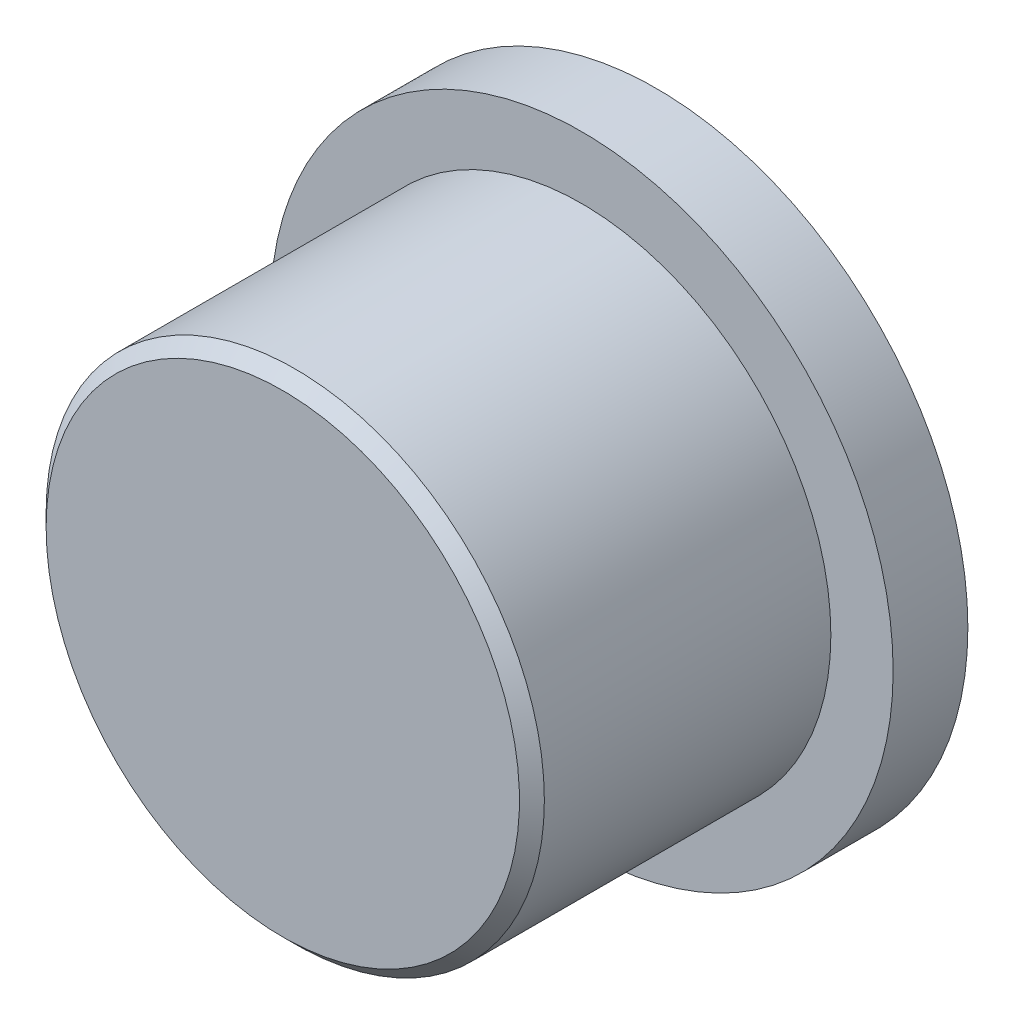
from build123d import *

# Parameters (mm, degrees)
CHAMFER1_SIZE = 0.5


with BuildPart() as part:
    # Sketch1 → Revolve1 (revolve)
    with BuildSketch(Plane(origin=(0, 0, 0), x_dir=(0, 0, -1), z_dir=(1, 0, 0)), mode=Mode.PRIVATE) as revolve1_sk:
        Polygon((15, 0), (15, 12.5), (12, 12.5), (12, 10), (0, 10), (0, 0), align=None)
    revolve(revolve1_sk.sketch.rotate(Axis((0, 0, 0), (0, 0, -1)), 90), axis=Axis((0, 0, 0), (0, 0, -1)))

    # Chamfer1
    chamfer1_edges = [part.edges().sort_by_distance(p)[0] for p in [
        (-10, 0, 0),
    ]]
    chamfer(chamfer1_edges, length=CHAMFER1_SIZE)


solid = part.part
